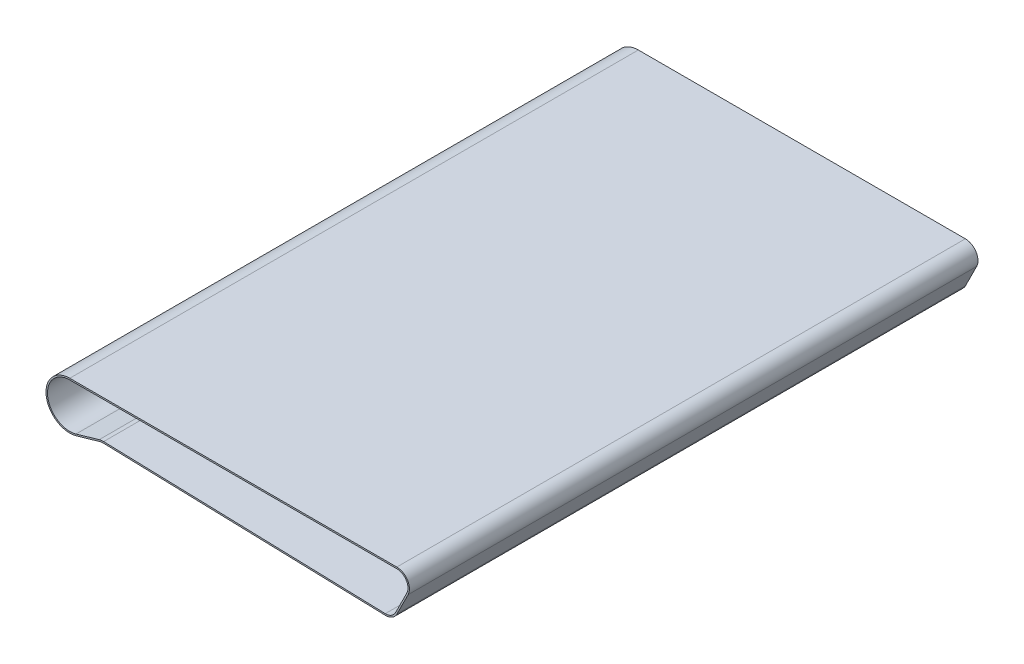
SolidWorks part; units mm, degrees
ref_plane "前视基准面" through (0, 0, 0) normal (0, 0, 1) x (1, 0, 0)
ref_plane "上视基准面" through (0, 0, 0) normal (0, 1, 0) x (1, 0, 0)
ref_plane "右视基准面" through (0, 0, 0) normal (1, 0, 0) x (0, 0, -1)
sketch "草图1" plane through (0, 0, 0) normal (0, 0, 1) x (1, 0, 0)
  line L8 (0, 30) -> (440, 30)
  line L9 (453.4164, 8.2918) -> (438.4164, -21.7082)
  line L10 (45.565, -19.0082) -> (424.5654, -29.9937)
  line L11 (8.3468, -28.8155) -> (39.5746, -19.7699)
  line L13 (8.9032, -30.7365) -> (40.1311, -21.691)
  line L14 (45.507, -21.0073) -> (424.5075, -31.9929)
  line L15 (455.2053, 7.3974) -> (440.2053, -22.6026)
  line L16 (0, 32) -> (440, 32)
  arc A2 (0, 32) -> (8.9032, -30.7365) centre (0, 0) ccw
  circle A4 centre (45, -38.5) radius 19.5
  arc A6 (45.565, -19.0082) -> (39.5746, -19.7699) centre (45, -38.5) ccw
  circle A12 centre (0, 0) radius 30 construction
  arc A13 (0, 30) -> (8.3468, -28.8155) centre (0, 0) ccw
  circle A16 centre (440, 15) radius 15 construction
  arc A17 (453.4164, 8.2918) -> (440, 30) centre (440, 15) ccw
  circle A18 centre (425, -15) radius 15 construction
  arc A19 (424.5654, -29.9937) -> (438.4164, -21.7082) centre (425, -15) ccw
  arc A20 (45.507, -21.0073) -> (40.1311, -21.691) centre (45, -38.5) ccw
  arc A21 (424.5075, -31.9929) -> (440.2053, -22.6026) centre (425, -15) ccw
  arc A22 (455.2053, 7.3974) -> (440, 32) centre (440, 15) ccw
  dimension "D1" = 2
  dimension "D2" = 2
extrude "凸台-拉伸1" add sketch "草图1" along normal mid plane 765
sketch "草图2" plane through (0, 0, 0) normal (0, 1, 0) x (1, 0, 0)
  line L1 (-728.0312, 15) -> (728.0312, 15)
  line L2 (-728.0312, 15) -> (-728.0312, -15)
  line L3 (-728.0312, -15) -> (728.0312, -15)
  line L4 (728.0312, 15) -> (728.0312, -15)
  line L5 (-728.0312, 15) -> (728.0312, -15) construction
  line L6 (-728.0312, -15) -> (728.0312, 15) construction
  point P0 (0, 0)
  dimension "D1" = 30
